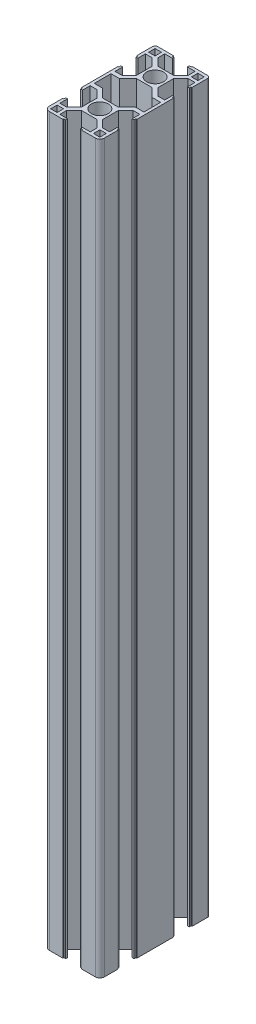
SolidWorks part; units mm, degrees
material "6063 alloy"
ref_plane "Front Plane" through (0, 0, 0) normal (0, 0, 1) x (1, 0, 0)
ref_plane "Top Plane" through (0, 0, 0) normal (0, 1, 0) x (1, 0, 0)
ref_plane "Right Plane" through (0, 0, 0) normal (1, 0, 0) x (0, 0, -1)
sketch "草图1" plane through (0, 0, 0) normal (0, 0, 1) x (1, 0, 0)
  line L0 (0, 0) -> (0, 395)
  dimension "D1" = 395
other "Aluminum profile 30 X 60L X R2.5(1)"
ref_plane "Plane1" through (0, 0, 0) normal (0, 1, 0) x (-1, 0, 0)
sketch "Sketch1" plane through (0, 0, 0) normal (0, 1, 0) x (-1, 0, 0)
  line L0 (-5.1, 15) -> (-5.1, 14.5)
  line L1 (-5.1, 14.5) -> (-4.1, 14.5)
  line L2 (-4.1, 14.5) -> (-4.1, 13.5)
  line L3 (-4.1, 13.5) -> (-8.25, 13.5)
  line L4 (8.9, -10.45) -> (4.25, -5.8)
  line L5 (-15, -24.9) -> (-15, -5.1)
  line L6 (12.5, 15) -> (5.1, 15)
  line L7 (15, 12.5) -> (15, 5.1)
  line L8 (0, 15) -> (0, 0) construction
  line L9 (0, 0) -> (15, 0) construction
  line L10 (-8.25, 13.5) -> (-8.25, 9.8)
  line L11 (-8.25, 9.8) -> (-4.25, 5.8)
  line L12 (-4.25, 5.8) -> (4.25, 5.8)
  line L13 (8.25, 9.8) -> (4.25, 5.8)
  line L14 (8.25, 13.5) -> (8.25, 9.8)
  line L15 (4.1, 13.5) -> (8.25, 13.5)
  line L16 (4.1, 14.5) -> (4.1, 13.5)
  line L17 (5.1, 14.5) -> (4.1, 14.5)
  line L18 (5.1, 15) -> (5.1, 14.5)
  line L19 (-5.1, 15) -> (-12.5, 15)
  line L20 (15, 5.1) -> (14.5, 5.1)
  line L21 (14.5, 5.1) -> (14.5, 4.1)
  line L22 (14.5, 4.1) -> (13.5, 4.1)
  line L23 (13.5, 4.1) -> (13.5, 8.25)
  line L24 (13.5, 8.25) -> (9.8, 8.25)
  line L25 (9.8, 8.25) -> (5.8, 4.25)
  line L26 (5.8, 4.25) -> (5.8, -4.25)
  line L27 (9.8, -8.25) -> (5.8, -4.25)
  line L28 (13.5, -8.25) -> (9.8, -8.25)
  line L29 (13.5, -4.1) -> (13.5, -8.25)
  line L30 (14.5, -4.1) -> (13.5, -4.1)
  line L31 (14.5, -5.1) -> (14.5, -4.1)
  line L32 (15, -5.1) -> (14.5, -5.1)
  line L33 (8.9, -19.55) -> (4.25, -24.2)
  line L34 (-8.9, -19.55) -> (-4.25, -24.2)
  line L35 (-8.9, -10.45) -> (-4.25, -5.8)
  line L36 (-13.5, -10.45) -> (-8.9, -10.45)
  line L37 (-13.5, -19.55) -> (-8.9, -19.55)
  line L38 (-13.5, -10.45) -> (-9.8, -10.45) construction
  line L39 (4.25, -5.8) -> (-4.25, -5.8)
  line L40 (-13.5, -19.55) -> (-9.8, -19.55) construction
  line L41 (-13.5, -10.45) -> (-13.5, -19.55)
  line L42 (13.5, -10.45) -> (13.5, -19.55)
  line L43 (8.9, -10.45) -> (13.5, -10.45)
  line L44 (8.9, -19.55) -> (13.5, -19.55)
  line L45 (-11.625, 11.625) -> (-11.625, 16.245) construction
  line L46 (-15, -5.1) -> (-14.5, -5.1)
  line L47 (-14.5, -5.1) -> (-14.5, -4.1)
  line L48 (-14.5, -4.1) -> (-13.5, -4.1)
  line L49 (-13.5, -4.1) -> (-13.5, -8.25)
  line L50 (-13.5, -8.25) -> (-9.8, -8.25)
  line L51 (-9.8, -8.25) -> (-5.8, -4.25)
  line L52 (-5.8, -4.25) -> (-5.8, 4.25)
  line L53 (-9.8, 8.25) -> (-5.8, 4.25)
  line L54 (-13.5, 8.25) -> (-9.8, 8.25)
  line L55 (-13.5, 4.1) -> (-13.5, 8.25)
  line L56 (-14.5, 4.1) -> (-13.5, 4.1)
  line L57 (-14.5, 5.1) -> (-14.5, 4.1)
  line L58 (-15, 5.1) -> (-14.5, 5.1)
  line L59 (-13.375, 13.375) -> (-9.875, 13.375)
  line L60 (-15, 5.1) -> (-15, 12.5)
  line L61 (15, -5.1) -> (15, -24.9)
  line L62 (-13.375, 13.375) -> (-13.375, 9.875)
  line L63 (-13.375, 9.875) -> (-9.875, 9.875)
  line L64 (-9.875, 13.375) -> (-9.875, 9.875)
  line L65 (-11.625, 11.625) -> (-7.4229, 11.625) construction
  line L66 (-13.5, -45) -> (-5.1, -45)
  line L67 (-15, -43.5) -> (-15, -35.1)
  line L68 (9.875, 13.375) -> (13.375, 13.375)
  line L69 (9.875, 13.375) -> (9.875, 9.875)
  line L70 (9.875, 9.875) -> (13.375, 9.875)
  line L71 (13.375, 13.375) -> (13.375, 9.875)
  line L72 (-4.25, -24.2) -> (4.25, -24.2)
  line L73 (-13.375, -39.875) -> (-9.875, -39.875)
  line L74 (-13.375, -39.875) -> (-13.375, -43.375)
  line L75 (-13.375, -43.375) -> (-9.875, -43.375)
  line L76 (-9.875, -39.875) -> (-9.875, -43.375)
  line L77 (9.875, -39.875) -> (13.375, -39.875)
  line L78 (9.875, -39.875) -> (9.875, -43.375)
  line L79 (9.875, -43.375) -> (13.375, -43.375)
  line L80 (15, -24.9) -> (14.5, -24.9)
  line L81 (14.5, -24.9) -> (14.5, -25.9)
  line L82 (14.5, -25.9) -> (13.5, -25.9)
  line L83 (13.5, -25.9) -> (13.5, -21.75)
  line L84 (13.5, -21.75) -> (9.8, -21.75)
  line L85 (9.8, -21.75) -> (5.8, -25.75)
  line L86 (5.8, -25.75) -> (5.8, -34.25)
  line L87 (9.8, -38.25) -> (5.8, -34.25)
  line L88 (13.5, -38.25) -> (9.8, -38.25)
  line L89 (13.5, -34.1) -> (13.5, -38.25)
  line L90 (14.5, -34.1) -> (13.5, -34.1)
  line L91 (14.5, -35.1) -> (14.5, -34.1)
  line L92 (15, -35.1) -> (14.5, -35.1)
  line L93 (5.1, -45) -> (5.1, -44.5)
  line L94 (5.1, -44.5) -> (4.1, -44.5)
  line L95 (4.1, -44.5) -> (4.1, -43.5)
  line L96 (4.1, -43.5) -> (8.25, -43.5)
  line L97 (8.25, -43.5) -> (8.25, -39.8)
  line L98 (8.25, -39.8) -> (4.25, -35.8)
  line L99 (4.25, -35.8) -> (-4.25, -35.8)
  line L100 (-8.25, -39.8) -> (-4.25, -35.8)
  line L101 (-8.25, -43.5) -> (-8.25, -39.8)
  line L102 (-4.1, -43.5) -> (-8.25, -43.5)
  line L103 (-4.1, -44.5) -> (-4.1, -43.5)
  line L104 (-5.1, -44.5) -> (-4.1, -44.5)
  line L105 (-5.1, -45) -> (-5.1, -44.5)
  line L106 (-15, -35.1) -> (-14.5, -35.1)
  line L107 (-14.5, -35.1) -> (-14.5, -34.1)
  line L108 (-14.5, -34.1) -> (-13.5, -34.1)
  line L109 (-13.5, -34.1) -> (-13.5, -38.25)
  line L110 (-13.5, -38.25) -> (-9.8, -38.25)
  line L111 (-9.8, -38.25) -> (-5.8, -34.25)
  line L112 (-5.8, -34.25) -> (-5.8, -25.75)
  line L113 (-9.8, -21.75) -> (-5.8, -25.75)
  line L114 (-13.5, -21.75) -> (-9.8, -21.75)
  line L115 (-13.5, -25.9) -> (-13.5, -21.75)
  line L116 (-14.5, -25.9) -> (-13.5, -25.9)
  line L117 (-14.5, -24.9) -> (-14.5, -25.9)
  line L118 (-15, -24.9) -> (-14.5, -24.9)
  line L119 (5.1, -45) -> (13.5, -45)
  line L120 (13.375, -39.875) -> (13.375, -43.375)
  line L121 (15, -35.1) -> (15, -43.5)
  line L122 (0, -30) -> (15, -30) construction
  line L125 (5.1, -15) -> (5.1, -14.5) [skipped]
  line L127 (5.1, -14.5) -> (4.1, -14.5) [skipped]
  line L129 (4.1, -14.5) -> (4.1, -13.5) [skipped]
  line L131 (4.1, -13.5) -> (8.25, -13.5) [skipped]
  line L133 (-4.1, -13.5) -> (-8.25, -13.5) [skipped]
  line L135 (-4.1, -14.5) -> (-4.1, -13.5) [skipped]
  line L137 (-5.1, -14.5) -> (-4.1, -14.5) [skipped]
  line L139 (-5.1, -15) -> (-5.1, -14.5) [skipped]
  line L141 (-5.1, -15) -> (-5.1, -15.5) [skipped]
  line L142 (-5.1, -15.5) -> (-4.1, -15.5) [skipped]
  line L143 (-4.1, -15.5) -> (-4.1, -16.5) [skipped]
  line L144 (-4.1, -16.5) -> (-8.25, -16.5) [skipped]
  line L145 (12.5, -15) -> (5.1, -15) [skipped]
  line L146 (4.1, -16.5) -> (8.25, -16.5) [skipped]
  line L147 (4.1, -15.5) -> (4.1, -16.5) [skipped]
  line L148 (5.1, -15.5) -> (4.1, -15.5) [skipped]
  line L149 (5.1, -15) -> (5.1, -15.5) [skipped]
  line L150 (-5.1, -15) -> (-12.5, -15) [skipped]
  line L151 (-15, -24.9) -> (-15, -17.5) [skipped]
  line L152 (15, -17.5) -> (15, -24.9) [skipped]
  line L154 (-8.25, -13.5) -> (-8.25, -9.8) [skipped]
  line L156 (8.25, -13.5) -> (8.25, -9.8) [skipped]
  line L157 (8.25, -16.5) -> (8.25, -20.2) [skipped]
  line L158 (-8.25, -16.5) -> (-8.25, -20.2) [skipped]
  line L160 (-12.5, -14.05) -> (-9.7895, -11.3395) [skipped]
  line L161 (18.444, -10.006) -> (14.8, -13.65) [skipped]
  line L163 (11.9857, -13.5357) -> (9.7894, -11.3394) [skipped]
  line L164 (-15.9344, -12.5156) -> (-14.8, -13.65) [skipped]
  line L165 (9.7894, -15) -> (-9.8, -15) construction
  circle A0 centre (0, 0) radius 4.6
  arc A1 (-15, 12.5) -> (-12.5, 15) centre (-12.5, 12.5) cw
  arc A2 (15, 12.5) -> (12.5, 15) centre (12.5, 12.5) ccw
  arc A3 (15, -43.5) -> (13.5, -45) centre (13.5, -43.5) cw
  arc A4 (-15, -43.5) -> (-13.5, -45) centre (-13.5, -43.5) ccw
  circle A5 centre (0, -30) radius 4.6
  arc A12 (-15, -17.5) -> (-12.5, -15) centre (-12.5, -17.5) cw [skipped]
  arc A13 (15, -17.5) -> (12.5, -15) centre (12.5, -17.5) ccw [skipped]
  point P0 (-10, 0)
  point P1 (10, 0)
  point P2 (0, 20)
  point P4 (0, 0)
  point P5 (0, 0)
  point P6 (-10, 0)
  point P7 (15, 15)
  point P8 (-15, 15)
  point P12 (-15, -15)
  point P13 (15, -15)
  point P15 (0, -10)
  point P16 (10, 0)
  point P36 (-15, 15)
  point P39 (15, 15)
  point P43 (-10, -30)
  point P44 (10, -30)
  point P88 (0, -30)
  point P89 (0, -30)
  point P90 (-10, -30)
  point P91 (10, -30)
  point P102 (15, -45)
  point P120 (-15, -45)
  point P121 (0, 0)
  dimension "D1" = 16.5
  dimension "D2" = 30
  dimension "D3" = 8.2
  dimension "D4" = 10.2
  dimension "D5" = 9.2
  dimension "D6" = 9.2
  dimension "D7" = 2.5
  dimension "D8" = 45
  dimension "D14" = 30
  dimension "D15" = 1.5
  dimension "D9" = 0.5
  dimension "D10" = 1
  dimension "D11" = 8.5
  dimension "D12" = 15
  dimension "D13" = 60
  dimension "D16" = 45
  dimension "D17" = 45
  dimension "D18" = 10.2
  dimension "D19" = 8.2
  dimension "D20" = 2.2
  dimension "D22" = 3.5
  dimension "D21" = 2.2
